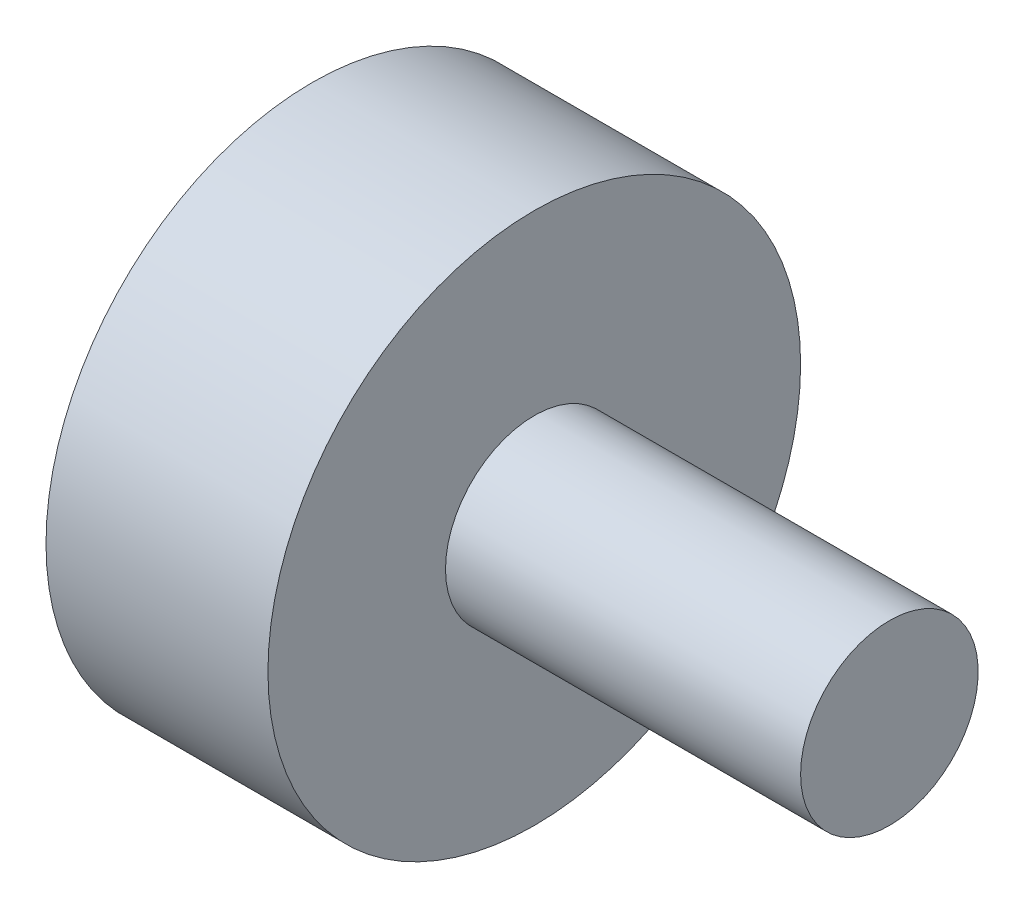
from build123d import *


with BuildPart() as part:
    # Sketch1 → Revolve1 (revolve)
    with BuildSketch(Plane.XY, mode=Mode.PRIVATE) as revolve1_sk:
        Polygon((0, 0), (0, 6), (5, 6), (5, 2), (13, 2), (13, 0), align=None)
    revolve(revolve1_sk.sketch.rotate(Axis((0, 0, 0), (1, 0, 0)), 90), axis=Axis((0, 0, 0), (1, 0, 0)))


solid = part.part
